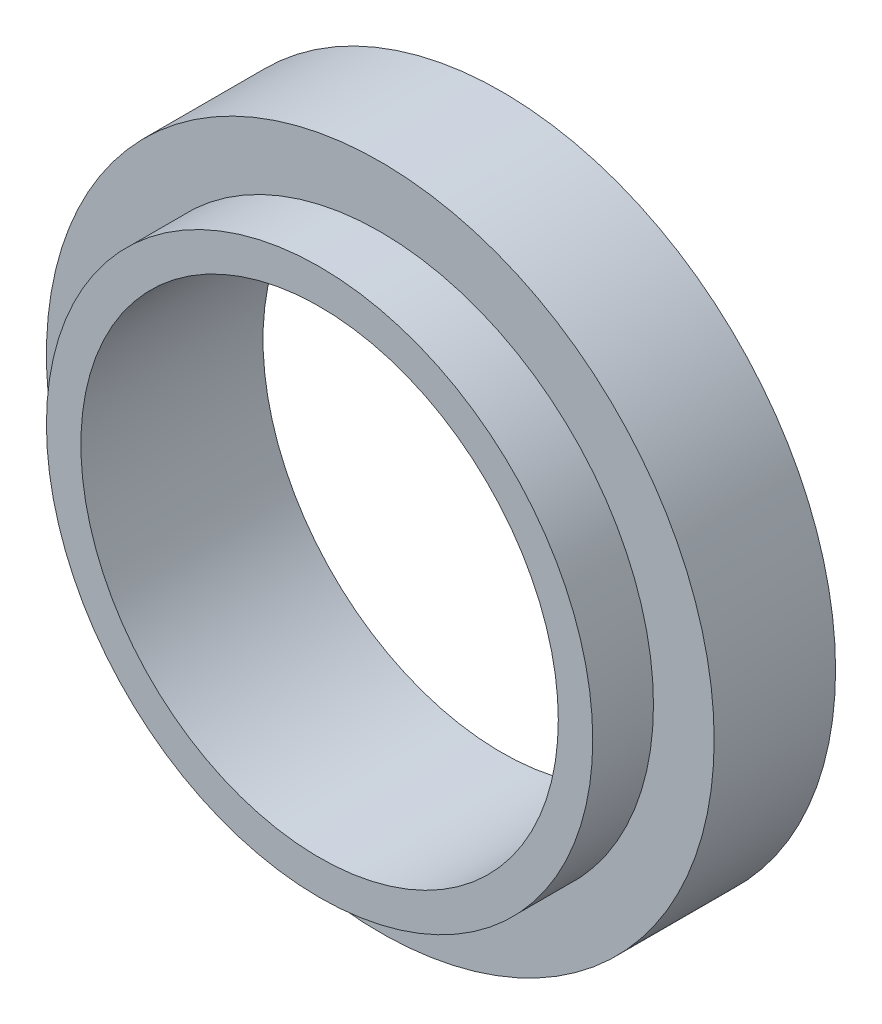
from build123d import *

# Parameters (mm, degrees)
SKETCH1_R           = 27.5
SKETCH1_R_2         = 19.662321429
BOSS_EXTRUDE1_DEPTH = 10
SKETCH2_R           = 22.5
SKETCH2_R_2         = 19.662321429
BOSS_EXTRUDE2_DEPTH = 5


with BuildPart() as part:
    # Sketch1 → Boss-Extrude1 (new body)
    with BuildSketch(Plane.XY):
        Circle(SKETCH1_R)
        Circle(SKETCH1_R_2, mode=Mode.SUBTRACT)
    extrude(amount=BOSS_EXTRUDE1_DEPTH)

    # Sketch2 → Boss-Extrude2 (add)
    with BuildSketch(Plane.XY.offset(10)):
        Circle(SKETCH2_R)
        Circle(SKETCH2_R_2, mode=Mode.SUBTRACT)
    extrude(amount=BOSS_EXTRUDE2_DEPTH)


solid = part.part
